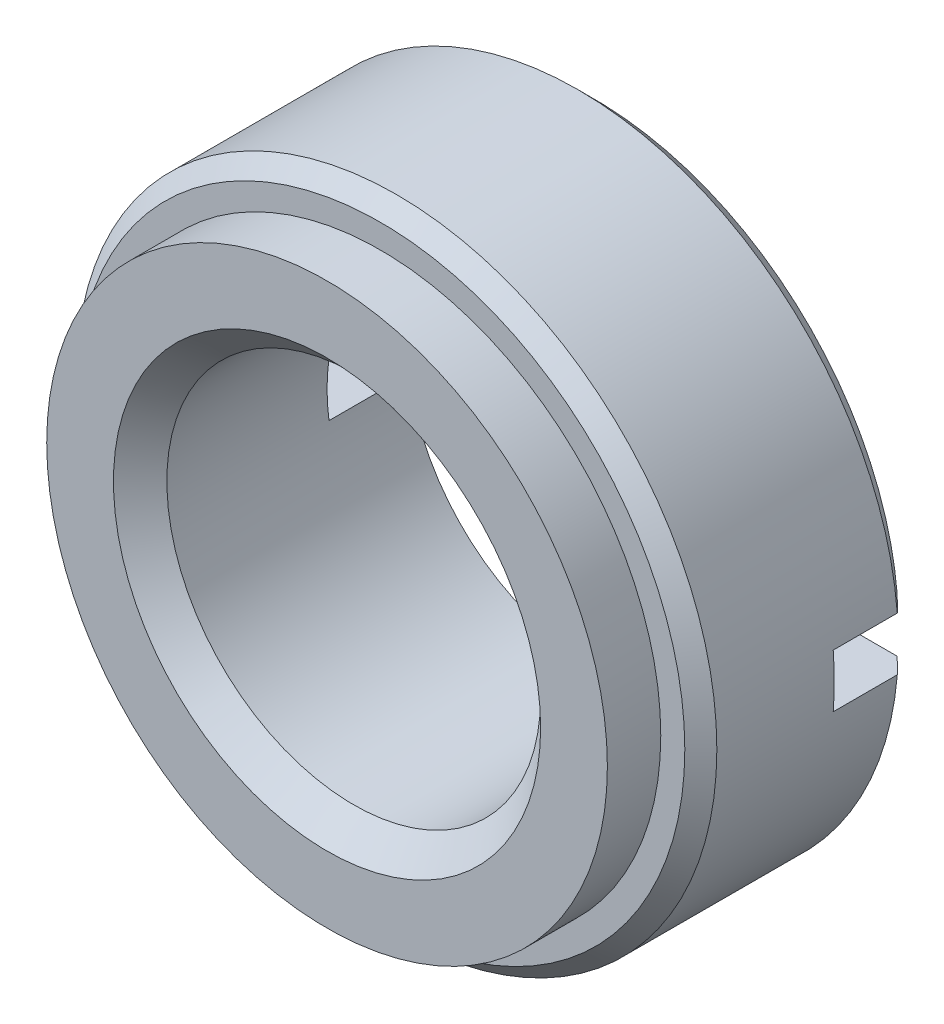
SolidWorks part; units mm, degrees
ref_plane "前视基准面" through (0, 0, 0) normal (0, 0, 1) x (1, 0, 0)
ref_plane "上视基准面" through (0, 0, 0) normal (0, 1, 0) x (1, 0, 0)
ref_plane "右视基准面" through (0, 0, 0) normal (1, 0, 0) x (0, 0, -1)
sketch "草图1" plane through (0, 0, 0) normal (0, 0, 1) x (1, 0, 0)
  circle A0 centre (0, 0) radius 6
  circle A1 centre (0, 0) radius 3.5
  dimension "D1" = 12
  dimension "D2" = 7
extrude "凸台-拉伸1" add sketch "草图1" along normal blind 5
cosmetic thread "装饰螺纹线6" parameters "D1"=4, "D2"=10.647
chamfer "倒角1" distance 0.5 angle 45 1 edges at (3.5, 0, 5)
sketch "草图2" plane through (0, 0, 0) normal (0, 0, -1) x (-1, 0, 0)
  line L0 (-8.7487, 0) -> (8.0925, 0) construction
  line L1 (-8.7487, -0.5) -> (8.0925, -0.5)
  line L2 (-8.7487, 0.5) -> (8.0925, 0.5)
  line L3 (-8.7487, 0.5) -> (-8.7487, -0.5)
  line L4 (8.0925, 0.5) -> (8.0925, -0.5)
  dimension "D1" = 0.5
  dimension "D2" = 0.5
extrude "切除-拉伸1" cut sketch "草图2" against normal blind 1.5
sketch "草图3" plane through (0, 0, 5) normal (0, 0, 1) x (1, 0, 0)
  circle A0 centre (0, 0) radius 5.25
  circle A1 centre (0, 0) radius 6
  dimension "D1" = 10.5
  dimension "D2" = 12
extrude "切除-拉伸2" cut sketch "草图3" against normal blind 1
chamfer "倒角2" distance 0.3 angle 45 3 edges at (0, 6, 0) (0, -6, 0) (6, 0, 4)
